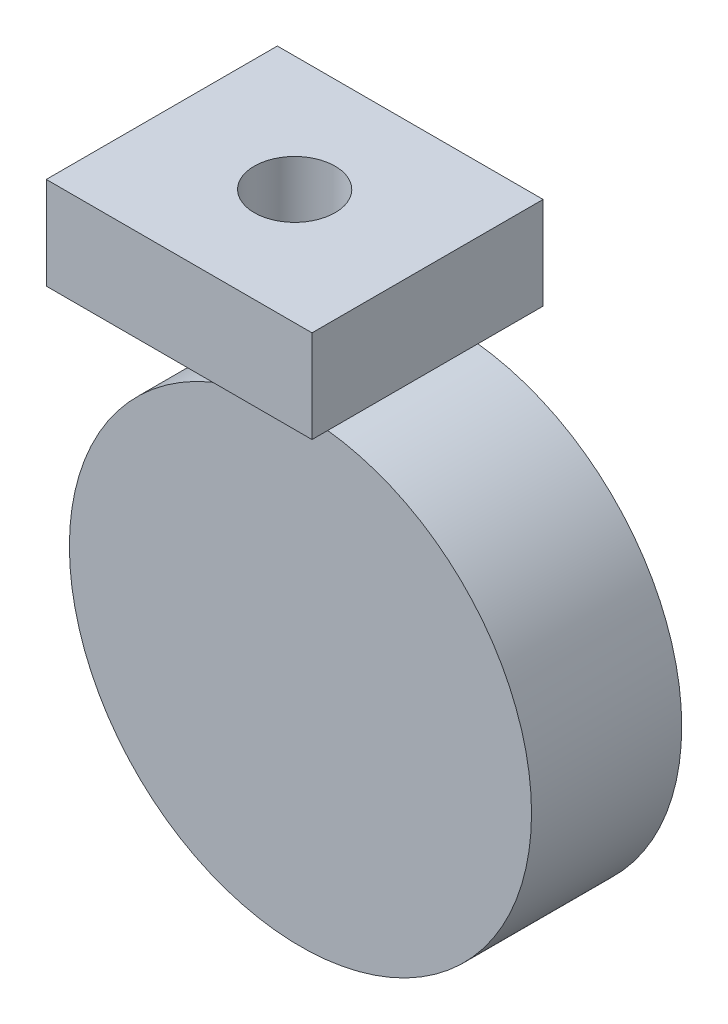
from build123d import *

# Parameters (mm, degrees)
SKETCH_1_R          = 100
EXTRUDE_1_DEPTH     = 32.5
SKETCH_2_W          = 115
SKETCH_2_H          = 40
EXTRUDE_2_DEPTH     = 50
SKETCH_3_R          = 17.480672493
CUT_EXTRUDE_1_DEPTH = 40


with BuildPart() as part:
    # 草图1 → 凸台-拉伸1 (new, symmetric)
    with BuildSketch(Plane.XY):
        Circle(SKETCH_1_R)
    extrude(amount=EXTRUDE_1_DEPTH, both=True)


with BuildPart() as body_2:
    # 草图2 → 凸台-拉伸2 (new, symmetric)
    with BuildSketch(Plane.XY):
        with Locations((-35, 130)):
            Rectangle(SKETCH_2_W, SKETCH_2_H)
    extrude(amount=EXTRUDE_2_DEPTH, both=True)

    # 草图3 → 切除-拉伸1 (cut)
    with BuildSketch(Plane(origin=(0, 150, 0), x_dir=(1, 0, 0), z_dir=(0, 1, 0))):
        with Locations(Location((-35, 0, 0), (0, 0, 270))):
            Circle(SKETCH_3_R)
    extrude(amount=-CUT_EXTRUDE_1_DEPTH, mode=Mode.SUBTRACT)


solid = Compound([part.part, body_2.part])
